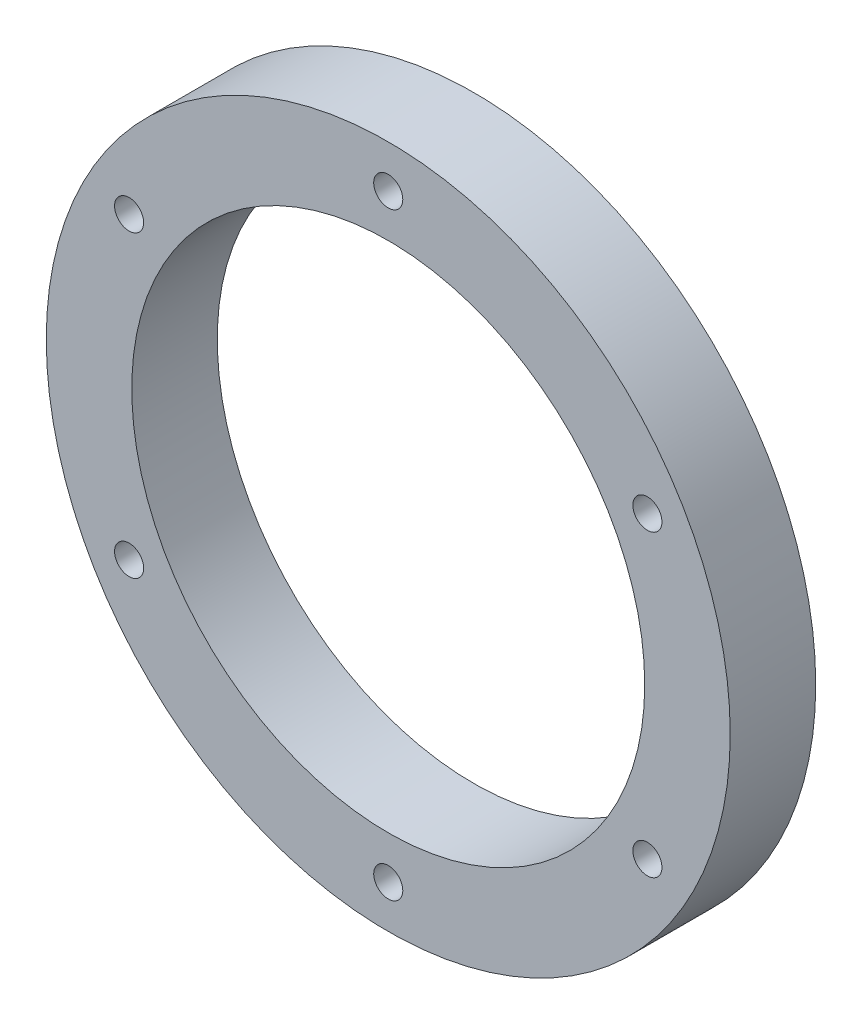
from build123d import *

# Parameters (mm, degrees)
SKETCH1_R             = 80
SKETCH1_R_2           = 60
BOSS_EXTRUDE1_DEPTH   = 20
M8_TAPPED_HOLE1_D     = 6.8
M8_TAPPED_HOLE1_DEPTH = 18
M8_TAPPED_HOLE1_TIP   = 2.042926105


with BuildPart() as part:
    # Sketch1 → Boss-Extrude1 (new body)
    with BuildSketch(Plane.XY):
        Circle(SKETCH1_R)
        Circle(SKETCH1_R_2, mode=Mode.SUBTRACT)
    extrude(amount=BOSS_EXTRUDE1_DEPTH)

    # M8 Tapped Hole1
    with Locations(Plane(origin=(0, 70, 20), x_dir=(1, 0, 0), z_dir=(0, 0, 1))):
        with Locations((0, 0), (60.621778265, -35), (60.621778265, -105), (0, -140), (-60.621778265, -105), (-60.621778265, -35)):
            Hole(M8_TAPPED_HOLE1_D / 2, depth=M8_TAPPED_HOLE1_DEPTH)
            with Locations((0, 0, -(M8_TAPPED_HOLE1_DEPTH + M8_TAPPED_HOLE1_TIP / 2))):  # 118° drill point
                Cone(0, M8_TAPPED_HOLE1_D / 2, M8_TAPPED_HOLE1_TIP, mode=Mode.SUBTRACT)


solid = part.part
